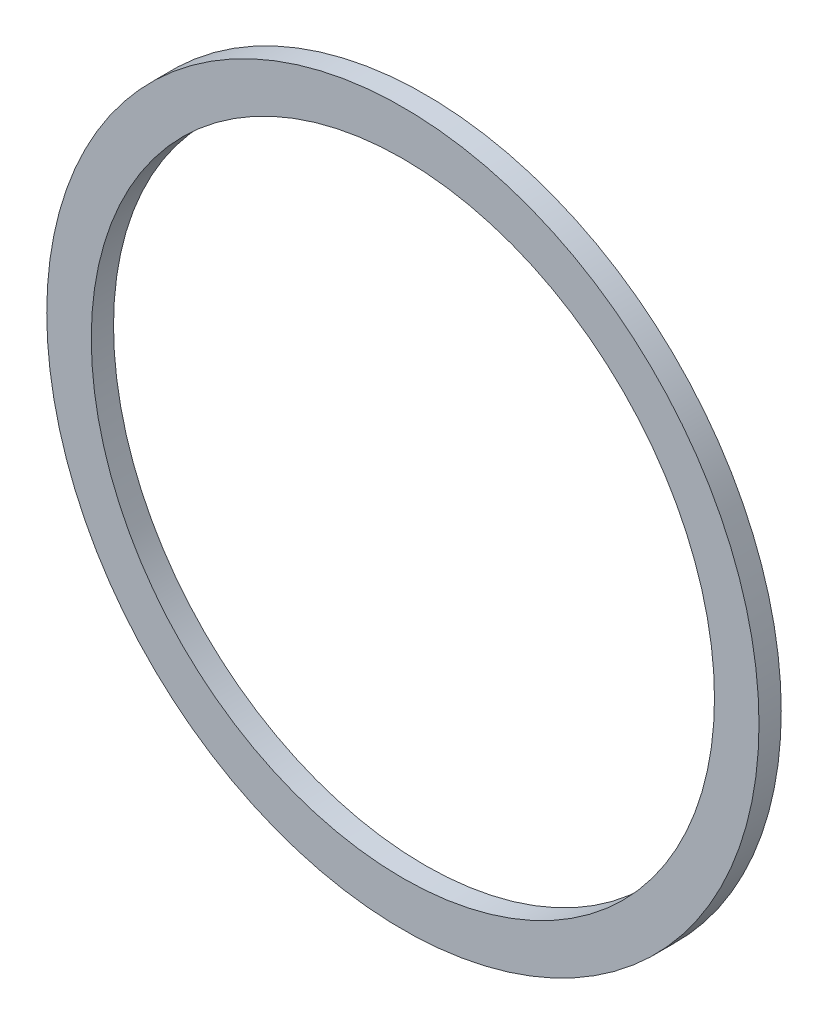
from build123d import *

# Parameters (mm, degrees)
SKETCH_1_R      = 40
SKETCH_1_R_2    = 35
EXTRUDE_1_DEPTH = 2.5


with BuildPart() as part:
    # 草图1 → 凸台-拉伸1 (new body)
    with BuildSketch(Plane.XY):
        Circle(SKETCH_1_R)
        Circle(SKETCH_1_R_2, mode=Mode.SUBTRACT)
    extrude(amount=EXTRUDE_1_DEPTH)


solid = part.part
